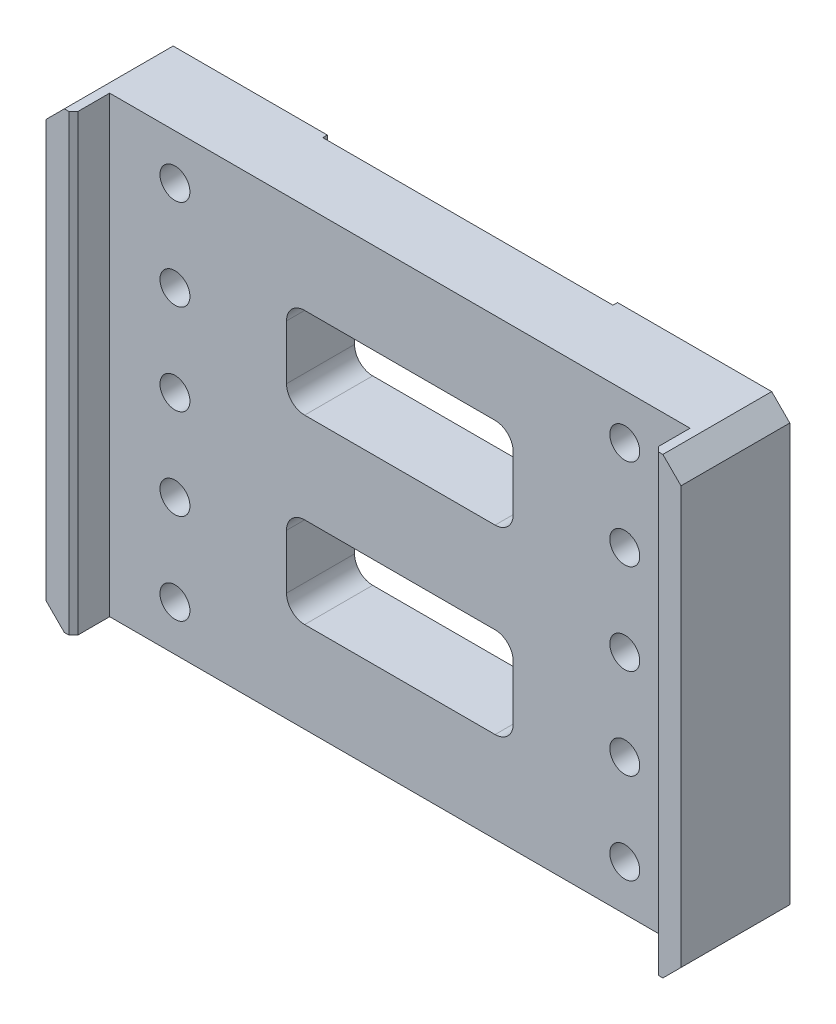
SolidWorks part; units mm, degrees
ref_plane "Front Plane" through (0, 0, 0) normal (0, 0, 1) x (1, 0, 0)
ref_plane "Top Plane" through (0, 0, 0) normal (0, 1, 0) x (1, 0, 0)
ref_plane "Right Plane" through (0, 0, 0) normal (1, 0, 0) x (0, 0, -1)
sketch "Sketch1" plane through (0, 0, 0) normal (0, 0, 1) x (1, 0, 0)
  line L1 (-35, -25) -> (35, -25)
  line L2 (-35, -25) -> (-35, 25)
  line L3 (-35, 25) -> (35, 25)
  line L4 (35, -25) -> (35, 25)
  line L5 (-35, -25) -> (35, 25) construction
  line L6 (-35, 25) -> (35, -25) construction
  point P0 (0, 0)
  dimension "D1" = 70
  dimension "D2" = 50
extrude "Boss-Extrude1" add sketch "Sketch1" along normal blind 12
sketch "Sketch2" plane through (0, -25, 0) normal (0, -1, 0) x (1, 0, 0)
  line L0 (-35, 12) -> (35, 12) construction
  line L1 (-32, 12) -> (32, 12)
  line L2 (-32, 12) -> (-32, 8)
  line L3 (-32, 8) -> (32, 8)
  line L4 (32, 12) -> (32, 8)
  line L5 (-35, 12) -> (-35, 0) construction
  line L6 (35, 12) -> (35, 0) construction
  dimension "D1" = 3
  dimension "D2" = 4
  dimension "D3" = 3
extrude "Cut-Extrude1" cut sketch "Sketch2" against normal through all
chamfer "Chamfer1" distance 0.5 angle 45 2 edges at (32, 0, 12) (-32, 0, 12)
sketch "Sketch3" plane through (0, 25, 0) normal (0, 1, 0) x (1, 0, 0)
  line L1 (16, 0) -> (-16, 0)
  line L2 (16, 0) -> (16, -0.5)
  line L3 (16, -0.5) -> (-16, -0.5)
  line L4 (-16, 0) -> (-16, -0.5)
  line L5 (16, -0.5) -> (16, 15.1) construction
  line L6 (-16, 11.1) -> (-16, -0.5) construction
  line L7 (35, 0) -> (-35, 0) construction
  dimension "D1" = 0.5
extrude "Cut-Extrude2" cut sketch "Sketch3" against normal through all
hole_wizard "M4 Tapped Hole1" positions "Sketch5" profile "Sketch6" tap size "M4" standard "GB"
sketch "Sketch5" plane through (0, 0, 8) normal (0, 0, 1) x (1, 0, 0)
  line L0 (-32, 25) -> (-32, -25) construction
  line L1 (-32, 25) -> (32, 25) construction
  point P0 (-24.8, 20)
  dimension "D1" = 7.2
  dimension "D2" = 5
sketch "Sketch6" plane through (-24.8, 20, 8) normal (1, 0, 0) x (0, -1, 0)
  line L0 (0, 0) -> (0, 12.4914)
  line L1 (0, 12.4914) -> (1.65, 11.5)
  line L2 (1.65, 11.5) -> (1.65, 0)
  line L5 (1.65, 0) -> (0, 0)
  line L10 (0, 12.4914) -> (-1.65, 11.5) construction
  line L11 (0, -6.35) -> (0, 107.95) construction
  dimension "螺纹孔钻头直径" = 3.3
  dimension "螺纹孔钻头深度" = 11.5
  dimension "导头角度" = 118
cosmetic thread "Cosmetic Thread1"
pattern_linear "LPattern1" count 5 spacing 10 along (0, -1, 0) of "M4 Tapped Hole1"
cosmetic thread "Cosmetic Thread2"
cosmetic thread "Cosmetic Thread3"
cosmetic thread "Cosmetic Thread4"
cosmetic thread "Cosmetic Thread5"
mirror "Mirror1" about plane through (0, 0, 0) normal (1, 0, 0) of "LPattern1", "M4 Tapped Hole1"
cosmetic thread "Cosmetic Thread6"
cosmetic thread "Cosmetic Thread7"
cosmetic thread "Cosmetic Thread8"
cosmetic thread "Cosmetic Thread9"
cosmetic thread "Cosmetic Thread10"
sketch "Sketch7" plane through (0, 0, 8) normal (0, 0, 1) x (1, 0, 0)
  line L0 (-32, -25) -> (32, -25) construction
  line L1 (-12.5, -5) -> (12.5, -5)
  line L2 (-12.5, -5) -> (-12.5, -15)
  line L3 (-12.5, -15) -> (12.5, -15)
  line L4 (12.5, -5) -> (12.5, -15)
  line L5 (0, 5) -> (0, -5) construction
  line L6 (0, 0) -> (-15.4964, 0) construction
  line L7 (12.5, 5) -> (12.5, 15)
  line L8 (-12.5, 15) -> (12.5, 15)
  line L9 (-12.5, 5) -> (-12.5, 15)
  line L10 (-12.5, 5) -> (12.5, 5)
  dimension "D1" = 10
  dimension "D2" = 10
  dimension "D3" = 25
extrude "Cut-Extrude3" cut sketch "Sketch7" against normal through all
fillet "Fillet1" radius 2 8 edges at (-12.5, -15, 4.25) (-12.5, -5, 4.25) (12.5, -5, 4.25) (12.5, -15, 4.25) (-12.5, 15, 4.25) (-12.5, 5, 4.25) (12.5, 5, 4.25) (12.5, 15, 4.25)
chamfer "Chamfer2" distance 2 angle 45 4 edges at (35, -25, 6) (-35, -25, 6) (-35, 25, 6) (35, 25, 6)
equation "\"1\"= \"代号代号\""
equation "\"2\"= \"名称代号\""
